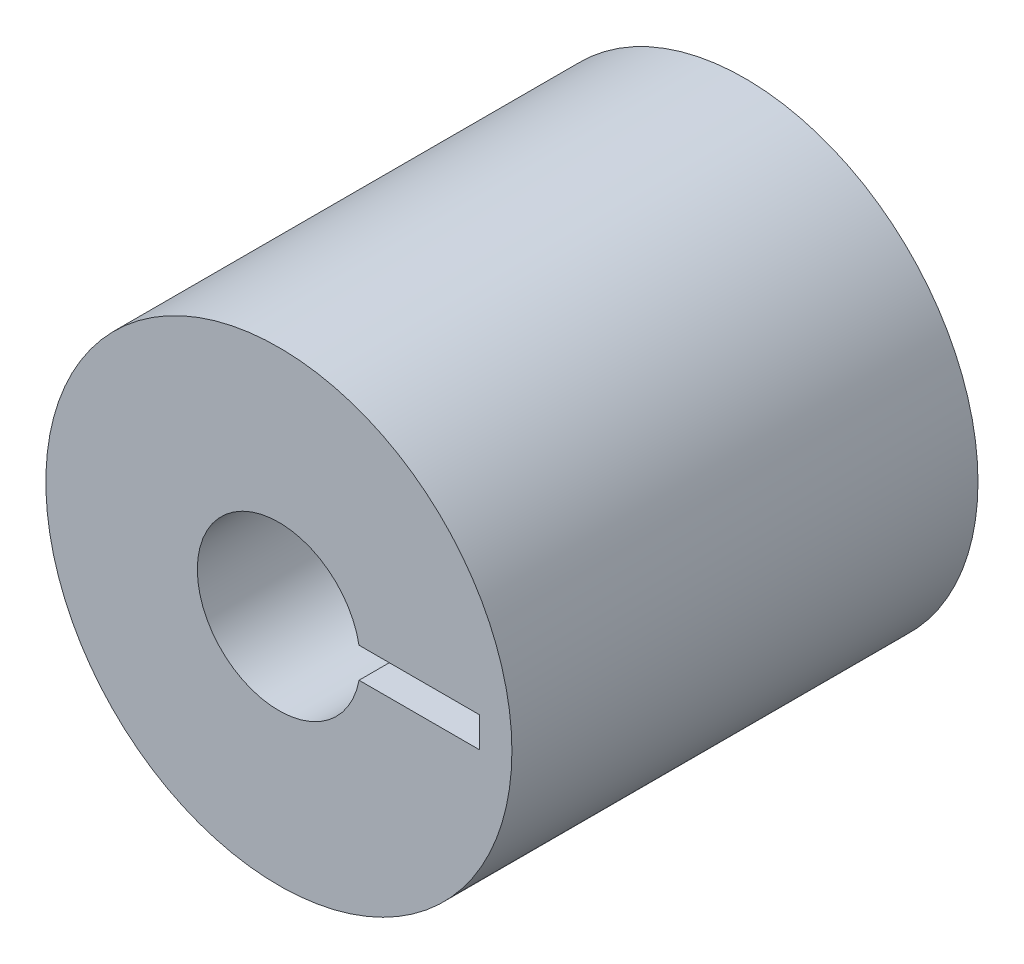
SolidWorks part; units mm, degrees
ref_plane "前视基准面" through (0, 0, 0) normal (0, 0, 1) x (1, 0, 0)
ref_plane "上视基准面" through (0, 0, 0) normal (0, 1, 0) x (1, 0, 0)
ref_plane "右视基准面" through (0, 0, 0) normal (1, 0, 0) x (0, 0, -1)
sketch "草图1" plane through (0, 0, 0) normal (0, 0, 1) x (1, 0, 0)
  circle A0 centre (0, 0) radius 20
  dimension "D1" = 40
extrude "凸台-拉伸1" add sketch "草图1" along normal blind 40
sketch "草图2" plane through (0, 0, 40) normal (0, 0, 1) x (1, 0, 0)
  circle A0 centre (0, 0) radius 4
  dimension "D1" = 8
extrude "切除-拉伸1" cut sketch "草图2" against normal through all
sketch "草图3" plane through (0, 0, 40) normal (0, 0, 1) x (1, 0, 0)
  circle A0 centre (0, 0) radius 7
  dimension "D1" = 14
extrude "切除-拉伸2" cut sketch "草图3" against normal blind 28
sketch "草图4" plane through (0, 0, 40) normal (0, 0, 1) x (1, 0, 0)
  line L0 (0, 0) -> (50000, 0) construction
  line L1 (17.2282, -1.3) -> (17.2282, 1.3)
  line L2 (17.2282, 1.3) -> (6.8782, 1.3)
  line L3 (17.2282, -1.3) -> (6.8782, -1.3)
  arc A0 (6.8782, -1.3) -> (6.8782, 1.3) centre (0, 0) ccw
  point P10 (17.2282, 0)
  dimension "D2" = 14
  dimension "D1" = 10.35
  dimension "D3" = 1.3
extrude "切除-拉伸3" cut sketch "草图4" against normal blind 13
sketch "草图5" plane through (0, 0, 0) normal (0, 0, -1) x (-1, 0, 0)
  line L0 (0, 0) -> (27.5669, 0) construction
  line L1 (16.9485, -0.64) -> (16.9485, 0.64)
  line L2 (16.9485, 0.64) -> (3.9485, 0.64)
  line L3 (16.9485, -0.64) -> (3.9485, -0.64)
  arc A0 (3.9485, -0.64) -> (3.9485, 0.64) centre (0, 0) ccw
  point P8 (16.9485, 0)
  dimension "D1" = 8
  dimension "D2" = 13
  dimension "D3" = 0.64
extrude "切除-拉伸4" cut sketch "草图5" against normal blind 13
